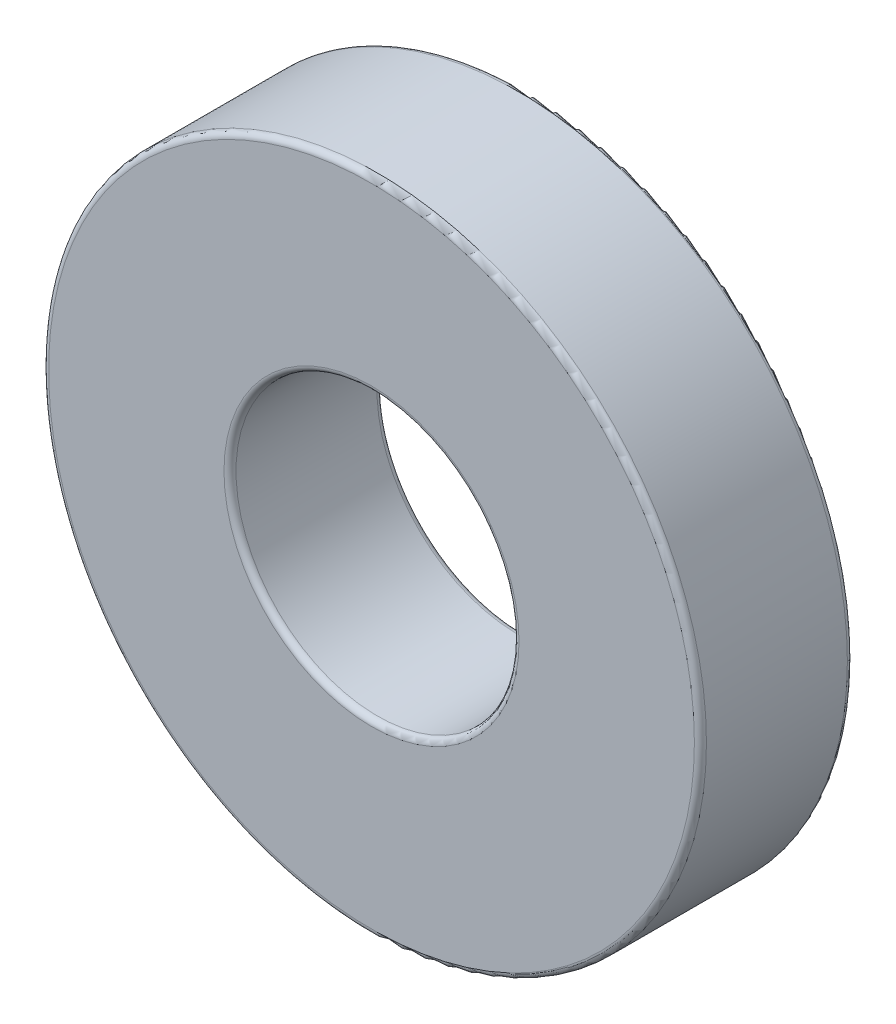
from build123d import *

# Parameters (mm, degrees)
SKETCH1_R           = 273.05
SKETCH1_R_2         = 117.475
BOSS_EXTRUDE1_DEPTH = 127
FILLET1_R           = 5


with BuildPart() as part:
    # Sketch1 → Boss-Extrude1 (new body)
    with BuildSketch(Plane.XY):
        Circle(SKETCH1_R)
        Circle(SKETCH1_R_2, mode=Mode.SUBTRACT)
    extrude(amount=BOSS_EXTRUDE1_DEPTH)

    # Fillet1
    fillet1_edges = [part.edges().sort_by_distance(p)[0] for p in [
        (-273.05, 0, 0),
        (-273.05, 0, 127),
        (-117.475, 0, 0),
        (-117.475, 0, 127),
    ]]
    fillet(fillet1_edges, radius=FILLET1_R)


solid = part.part
